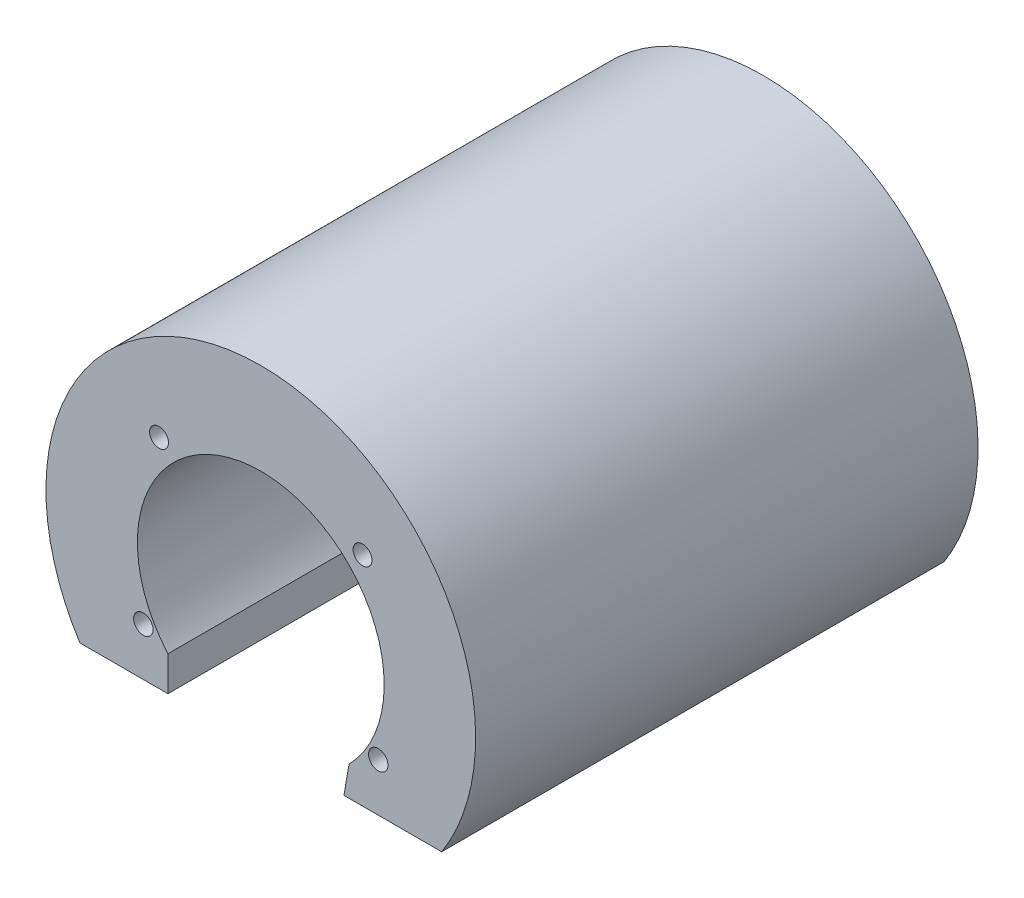
from build123d import *

# Parameters (mm, degrees)
SKETCH1_R           = 8
SKETCH1_R_2         = 8.25
BOSS_EXTRUDE1_DEPTH = 426


with BuildPart() as part:
    # Sketch1 → Boss-Extrude1 (new body)
    with BuildSketch(Plane.XY):
        with BuildLine():
            Line((-189.997809191, -121.602817484), (-189.997809191, -92.231705942))
            ThreePointArc((-189.997809191, -92.231705942), (-108.380706485, 81.229274354), (-36.431596452, -96.459748112))
            Line((-36.431596452, -96.459748112), (-40.758896177, -121.602817484))
            Line((-40.758896177, -121.602817484), (42.120800042, -121.602817484))
            ThreePointArc((42.120800042, -121.602817484), (-111.259960397, 158.805233349), (-264.640720837, -121.602817484))
            Line((-264.640720837, -121.602817484), (-189.997809191, -121.602817484))
        make_face()
        with Locations((-24.992933093, 62.919265507)):
            Circle(SKETCH1_R, mode=Mode.SUBTRACT)
        with Locations((-197.526987702, 62.919265507)):
            Circle(SKETCH1_R, mode=Mode.SUBTRACT)
        with Locations((-210.852881833, -80.847761798)):
            Circle(SKETCH1_R_2, mode=Mode.SUBTRACT)
        with Locations((-11.667038962, -80.847761798)):
            Circle(SKETCH1_R_2, mode=Mode.SUBTRACT)
    extrude(amount=-BOSS_EXTRUDE1_DEPTH)


solid = part.part
